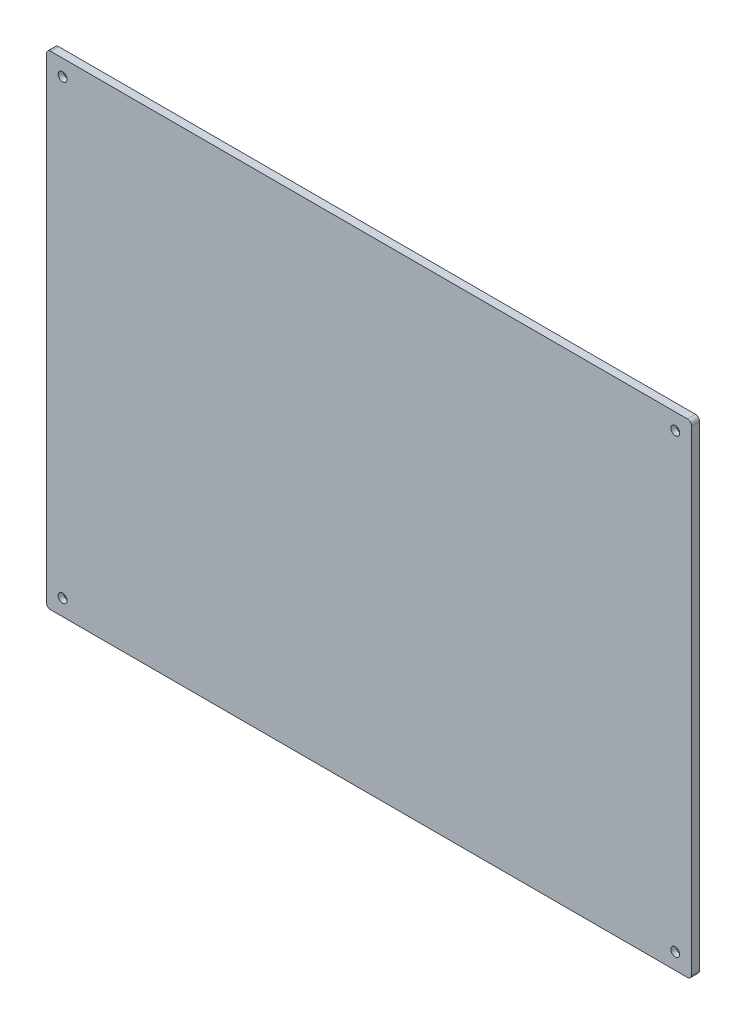
SolidWorks part; units mm, degrees
ref_plane "前视基准面" through (0, 0, 0) normal (0, 0, 1) x (1, 0, 0)
ref_plane "上视基准面" through (0, 0, 0) normal (0, 1, 0) x (1, 0, 0)
ref_plane "右视基准面" through (0, 0, 0) normal (1, 0, 0) x (0, 0, -1)
sketch "草图1" plane through (0, 0, 0) normal (0, 0, 1) x (1, 0, 0)
  line L1 (-400, 300) -> (400, 300)
  line L2 (-400, 300) -> (-400, -300)
  line L3 (-400, -300) -> (400, -300)
  line L4 (400, 300) -> (400, -300)
  line L5 (-400, 300) -> (400, -300) construction
  line L6 (-400, -300) -> (400, 300) construction
  point P0 (0, 0)
  dimension "D1" = 800
  dimension "D2" = 600
extrude "凸台-拉伸1" add sketch "草图1" along normal blind 10
hole_wizard "M6 六角凹头螺钉的柱形沉头孔1" positions "草图2" profile "草图4" counterbore size "M6" standard "ISO" end condition through all
sketch "草图2" plane through (0, 0, 10) normal (0, 0, 1) x (1, 0, 0)
  line L0 (400, 300) -> (-400, 300) construction
  line L1 (-400, 300) -> (-400, -300) construction
  line L2 (400, -300) -> (400, 300) construction
  line L3 (-400, -300) -> (400, -300) construction
  point P0 (-380, 280)
  point P2 (380, 280)
  point P4 (380, -280)
  point P6 (-380, -280)
  dimension "D1" = 20
  dimension "D2" = 20
  dimension "D3" = 20
  dimension "D4" = 20
sketch "草图4" plane through (-380, 280, 10) normal (1, 0, 0) x (0, -1, 0)
  line L0 (0, 0) -> (0, 10)
  line L1 (0, 10) -> (3.3, 10)
  line L3 (3.3, 10) -> (3.3, 6.4)
  line L4 (3.3, 6.4) -> (5.5, 6.4)
  line L5 (5.5, 6.4) -> (5.5, 0)
  line L7 (5.5, 0) -> (0, 0)
  line L11 (0, -6.35) -> (0, 107.95) construction
  dimension "通孔孔直径" = 6.6
  dimension "通孔孔深度" = 10
  dimension "柱形沉头孔直径" = 11
  dimension "柱形沉头孔深度" = 6.4
fillet "圆角1" radius 5 4 edges at (400, 300, 5) (400, -300, 5) (-400, -300, 5) (-400, 300, 5)
